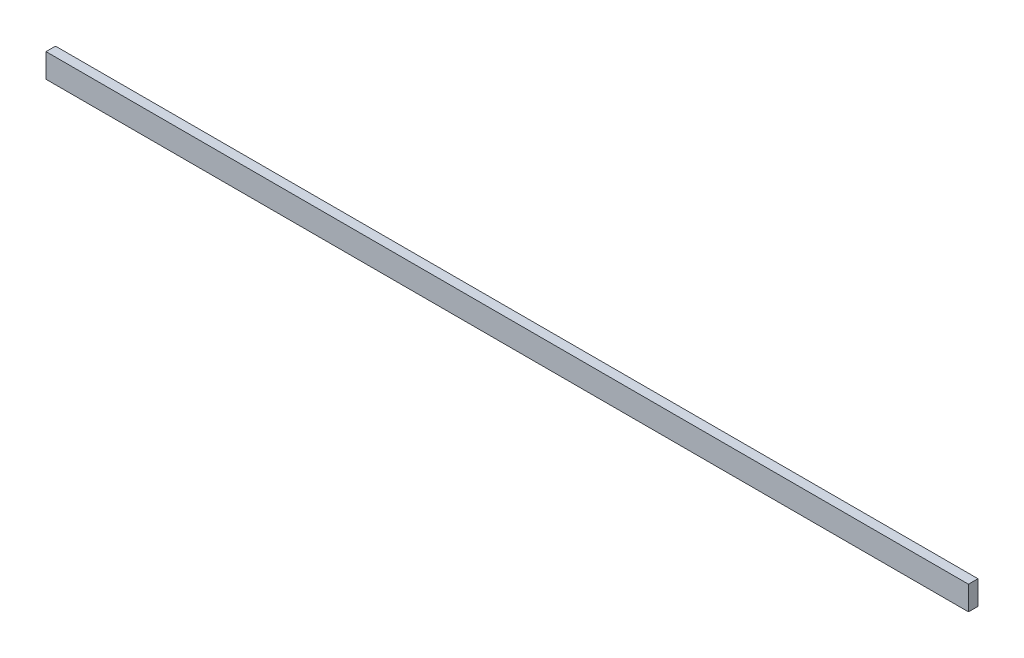
SolidWorks part; units mm, degrees
ref_plane "Front Plane" through (0, 0, 0) normal (0, 0, 1) x (1, 0, 0)
ref_plane "Top Plane" through (0, 0, 0) normal (0, 1, 0) x (1, 0, 0)
ref_plane "Right Plane" through (0, 0, 0) normal (1, 0, 0) x (0, 0, -1)
sketch "Sketch1" plane through (0, 0, 0) normal (0, 0, 1) x (1, 0, 0)
  line L1 (0, 0) -> (2425, 0)
  line L2 (0, 0) -> (0, 63)
  line L3 (0, 63) -> (2425, 63)
  line L4 (2425, 0) -> (2425, 63)
  dimension "D1" = 2425
  dimension "D2" = 63
extrude "Boss-Extrude1" add sketch "Sketch1" along normal blind 25
